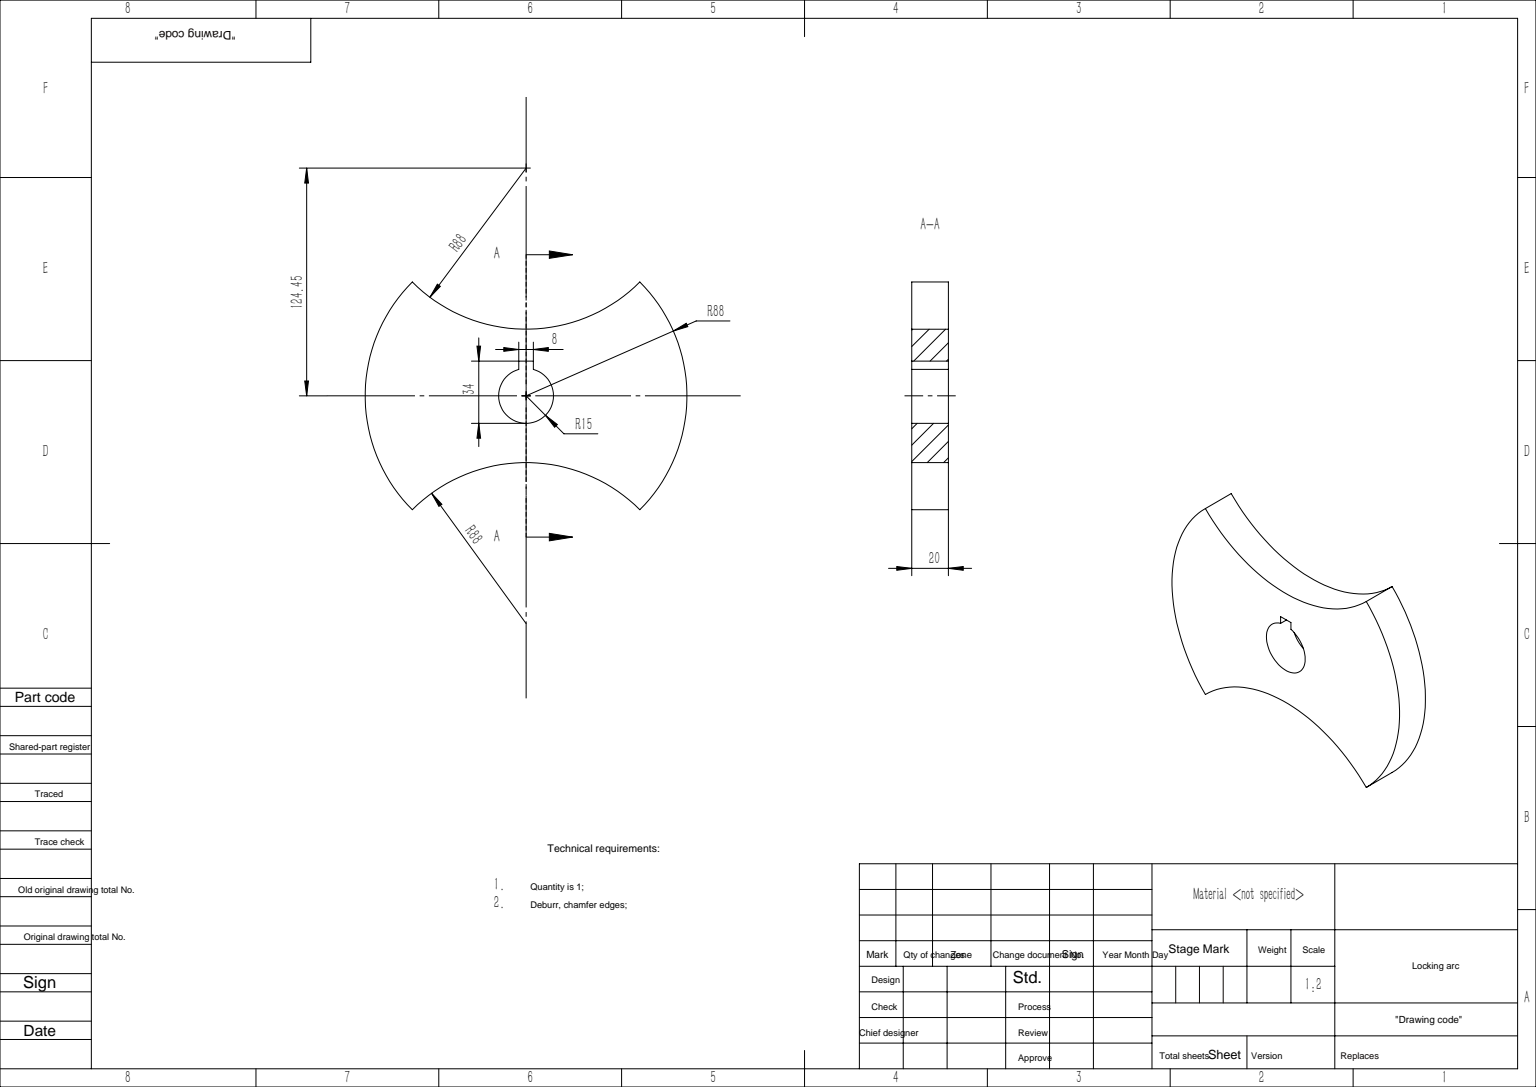
from build123d import *

# Parameters (mm, degrees)
EXTRUDE_1_DEPTH     = 20
CUT_EXTRUDE_1_DEPTH = 110.617516848


with BuildPart() as part:
    # 草图1 → 凸台-拉伸1 (new body)
    with BuildSketch(Plane.XY):
        with BuildLine():
            ThreePointArc((-62.225396744, 62.225396744), (-88, 0), (-62.225396744, -62.225396744))
            ThreePointArc((-62.225396744, -62.225396744), (0, -36.450793489), (62.225396744, -62.225396744))
            ThreePointArc((62.225396744, -62.225396744), (88, 0), (62.225396744, 62.225396744))
            ThreePointArc((62.225396744, 62.225396744), (0, 36.450793489), (-62.225396744, 62.225396744))
        make_face()
    extrude(amount=EXTRUDE_1_DEPTH)

    # 草图2 → 切除-拉伸1 (cut, through all)
    with BuildSketch(Plane.XY.offset(20)):
        with BuildLine():
            Line((-4, 19), (4, 19))
            Line((4, 19), (4, 14.456832295))
            ThreePointArc((4, 14.456832295), (0, -15), (-4, 14.456832295))
            Line((-4, 14.456832295), (-4, 19))
        make_face()
    extrude(amount=-CUT_EXTRUDE_1_DEPTH, mode=Mode.SUBTRACT)


solid = part.part
